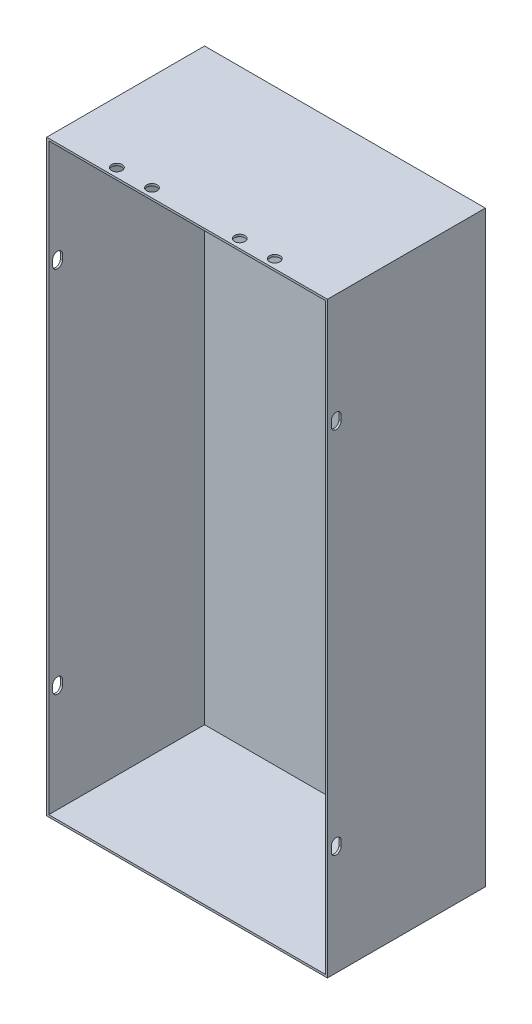
from build123d import *

# Parameters (mm, degrees)
SKETCH1_W           = 160
SKETCH1_H           = 335
BOSS_EXTRUDE1_DEPTH = 90
SHELL1_T            = -1.2
SKETCH2_R           = 3
CUT_EXTRUDE1_DEPTH  = 10
CUT_EXTRUDE2_DEPTH  = 249.508048159


with BuildPart() as part:
    # Sketch1 → Boss-Extrude1 (new body)
    with BuildSketch(Plane.XY):
        Rectangle(SKETCH1_W, SKETCH1_H)
    extrude(amount=BOSS_EXTRUDE1_DEPTH)

    # Shell1
    shell1_openings = [part.faces().sort_by_distance(p)[0] for p in [
        (0, 0, 90),
    ]]
    offset(amount=SHELL1_T, openings=shell1_openings, kind=Kind.INTERSECTION)

    # Sketch2 → Cut-Extrude1 (cut)
    with BuildSketch(Plane(origin=(0, 167.5, 0), x_dir=(1, 0, 0), z_dir=(0, 1, 0))):
        with Locations(Location((-45, -85, 0), (0, 0, 270))):
            Circle(SKETCH2_R)
        with Locations(Location((-25, -85, 0), (0, 0, 270))):
            Circle(SKETCH2_R)
        with Locations(Location((25, -85, 0), (0, 0, 270))):
            Circle(SKETCH2_R)
        with Locations(Location((45, -85, 0), (0, 0, 270))):
            Circle(SKETCH2_R)
    extrude(amount=-CUT_EXTRUDE1_DEPTH, mode=Mode.SUBTRACT)

    # Sketch3 → Cut-Extrude2 (cut, through all)
    with BuildSketch(Plane.ZY.offset(80)):
        with BuildLine():
            Line((87.8, 106.5), (87.8, 103.5))
            ThreePointArc((87.8, 103.5), (85, 100.7), (82.2, 103.5))
            Line((82.2, 103.5), (82.2, 106.5))
            ThreePointArc((82.2, 106.5), (85, 109.3), (87.8, 106.5))
        make_face()
        with BuildLine():
            Line((87.8, -106.5), (87.8, -103.5))
            ThreePointArc((87.8, -103.5), (85, -100.7), (82.2, -103.5))
            Line((82.2, -103.5), (82.2, -106.5))
            ThreePointArc((82.2, -106.5), (85, -109.3), (87.8, -106.5))
        make_face()
    extrude(amount=-CUT_EXTRUDE2_DEPTH, mode=Mode.SUBTRACT)


solid = part.part
